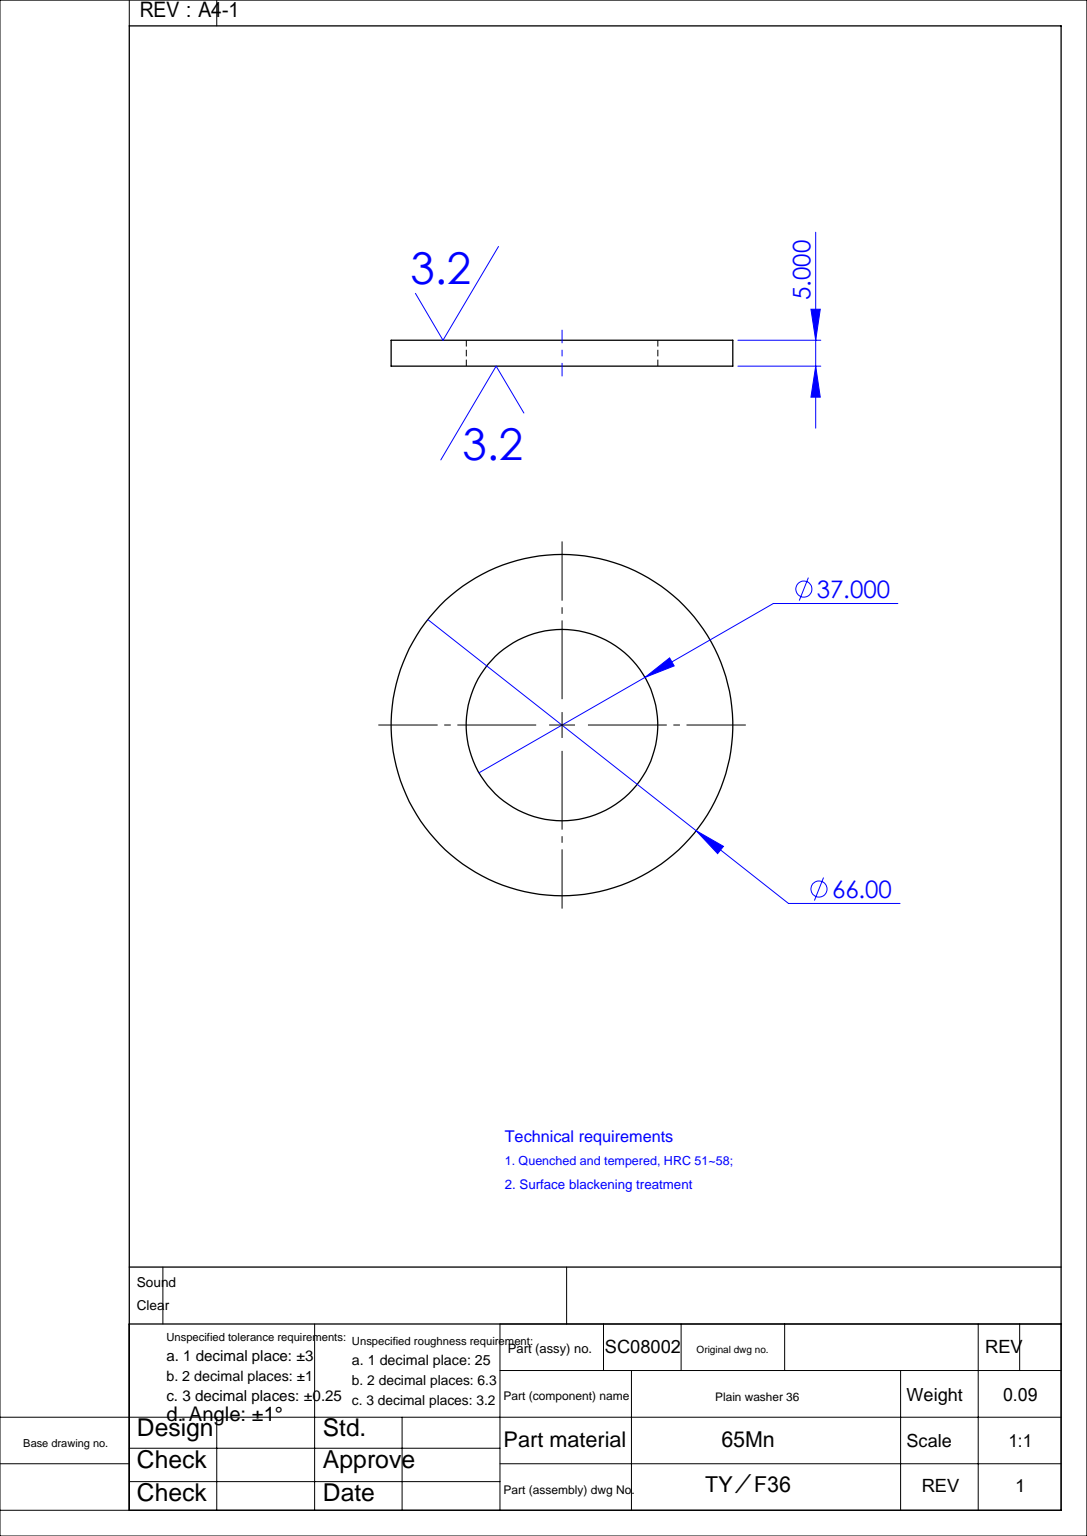
from build123d import *

# Parameters (mm, degrees)
SKETCH1_W = 14.5
SKETCH1_H = 5


with BuildPart() as part:
    # Sketch1 → Base-Revolve (revolve)
    with BuildSketch(Plane.XY, mode=Mode.PRIVATE) as base_revolve_sk:
        with Locations((-25.75, 11.144507042)):
            Rectangle(SKETCH1_W, SKETCH1_H)
    revolve(base_revolve_sk.sketch.rotate(Axis((0, 0, 0), (0, 1, 0)), 270), axis=Axis((0, 0, 0), (0, 1, 0)))


solid = part.part
